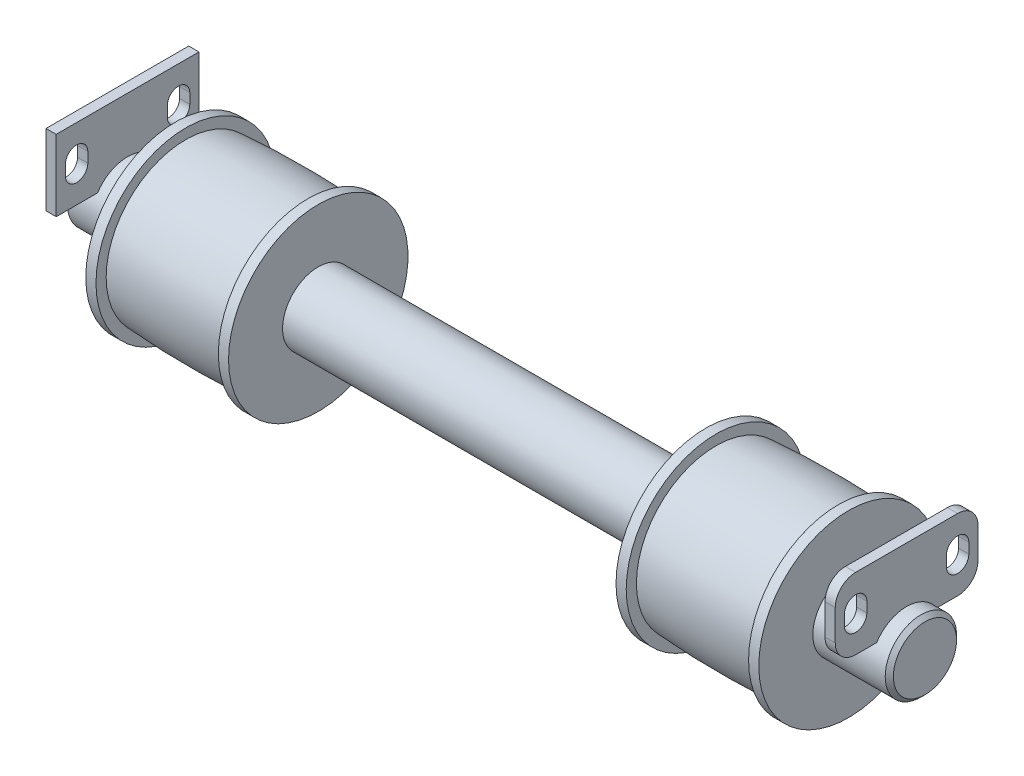
from build123d import *

# Parameters (mm, degrees)
CUT_EXTRUDE_1_DEPTH      = 72379.34823682
CUT_EXTRUDE_1_DEPTH_BACK = 72379.34823682
SKETCH_2_W               = 5
SKETCH_2_H               = 25.766795942
SKETCH_3_W               = 5
SKETCH_3_H               = 70
EXTRUDE_1_DEPTH          = 35
EXTRUDE_1_2_DEPTH        = 35
FILLET_1_R               = 10
CUT_EXTRUDE_2_DEPTH      = 4056.222125419
CUT_EXTRUDE_2_DEPTH_BACK = 4056.222125419


with BuildPart() as part:
    # 草图1 → 旋转1 (revolve)
    with BuildSketch(Plane.XY, mode=Mode.PRIVATE) as revolve_1_sk:
        with BuildLine():
            Line((72263.740728259, -3974.100882952), (72228.240728259, -3974.100882952))
            Line((72228.240728259, -3974.100882952), (72228.240728259, -3947.600882952))
            Line((72228.240728259, -3947.600882952), (72223.240728259, -3947.600882952))
            Line((72223.240728259, -3947.600882952), (72223.240728258, -3952.600882952))
            ThreePointArc((72223.240728258, -3952.600882952), (72193.240728259, -3951.600882952), (72163.240728259, -3952.600882952))
            Line((72163.240728259, -3952.600882952), (72163.240728259, -3947.600882952))
            Line((72163.240728259, -3947.600882952), (72158.240728259, -3947.600882952))
            Line((72158.240728259, -3947.600882952), (72158.240728259, -3974.100882952))
            Line((72158.240728259, -3974.100882952), (71968.240728259, -3974.100882952))
            Line((71968.240728259, -3974.100882952), (71968.240728259, -3947.600882952))
            Line((71968.240728259, -3947.600882952), (71963.240728259, -3947.600882952))
            Line((71963.240728259, -3947.600882952), (71963.240728258, -3952.600882952))
            ThreePointArc((71963.240728258, -3952.600882952), (71933.240728259, -3951.600882952), (71903.240728259, -3952.600882952))
            Line((71903.240728259, -3952.600882952), (71903.240728259, -3947.600882952))
            Line((71903.240728259, -3947.600882952), (71898.240728259, -3947.600882952))
            Line((71898.240728259, -3947.600882952), (71898.240728259, -3974.100882952))
            Line((71898.240728259, -3974.100882952), (71862.740728259, -3974.100882952))
            Line((71862.740728259, -3974.100882952), (71860.740728259, -3976.100882952))
            Line((71860.740728259, -3976.100882952), (71860.740728259, -3991.600882952))
            Line((71860.740728259, -3991.600882952), (72265.740728259, -3991.600882952))
            Line((72265.740728259, -3991.600882952), (72265.740728259, -3976.100882952))
            Line((72265.740728259, -3976.100882952), (72263.740728259, -3974.100882952))
        make_face()
    revolve(revolve_1_sk.sketch.rotate(Axis((71860.740728259, -3991.600882952, 0), (1, 0, 0)), 90), axis=Axis((71860.740728259, -3991.600882952, 0), (1, 0, 0)))

    # 草图2 → 切除-拉伸1 (cut, two sides: drawn at the far end of the back side and taken through both)
    with BuildSketch(Plane.XY.offset(-CUT_EXTRUDE_1_DEPTH_BACK)):
        with Locations((72254.240728259, -3969.217484981)):
            Rectangle(SKETCH_2_W, SKETCH_2_H)
        with Locations((71872.240728259, -3969.217484981)):
            Rectangle(SKETCH_2_W, SKETCH_2_H)
    extrude(amount=CUT_EXTRUDE_1_DEPTH + CUT_EXTRUDE_1_DEPTH_BACK, mode=Mode.SUBTRACT)


with BuildPart() as body_2:
    # 草图3 → 凸台-拉伸1 (new body)
    with BuildSketch(Plane(origin=(0, -3982.100882952, 0), x_dir=(1, 0, 0), z_dir=(0, 1, 0))):
        with Locations((72254.240728259, 0)):
            Rectangle(SKETCH_3_W, SKETCH_3_H)
    extrude(amount=EXTRUDE_1_DEPTH)

    # 圆角1
    fillet_1_edges = [body_2.edges().sort_by_distance(p)[0] for p in [
        (72254.240728259, -3947.100882952, -35),
        (72254.240728259, -3982.100882952, -35),
        (72254.240728259, -3982.100882952, 35),
        (72254.240728259, -3947.100882952, 35),
    ]]
    fillet(fillet_1_edges, radius=FILLET_1_R)


with BuildPart() as body_3:
    # 草图3 → Extrude 1 2 (new body)
    with BuildSketch(Plane(origin=(0, -3982.100882952, 0), x_dir=(1, 0, 0), z_dir=(0, 1, 0))):
        with Locations((71872.240728259, 0)):
            Rectangle(SKETCH_3_W, SKETCH_3_H)
    extrude(amount=EXTRUDE_1_2_DEPTH)


with BuildPart() as cut_extrude_2_tool:
    # 草图4 → 切除-拉伸2 (new, two sides: drawn at the far end of the back side and taken through both)
    with BuildSketch(Plane(origin=(72256.740728259, 0, 0), x_dir=(0, 0, -1), z_dir=(1, 0, 0)).offset(-CUT_EXTRUDE_2_DEPTH_BACK)):
        with BuildLine():
            Line((-19.5, -3962.100882952), (-19.5, -3967.100882952))
            ThreePointArc((-19.5, -3967.100882952), (-25, -3972.600882952), (-30.5, -3967.100882952))
            Line((-30.5, -3967.100882952), (-30.5, -3962.100882952))
            ThreePointArc((-30.5, -3962.100882952), (-25, -3956.600882952), (-19.5, -3962.100882952))
        make_face()
        with BuildLine():
            Line((19.5, -3962.100882952), (19.5, -3967.100882952))
            ThreePointArc((19.5, -3967.100882952), (25, -3972.600882952), (30.5, -3967.100882952))
            Line((30.5, -3967.100882952), (30.5, -3962.100882952))
            ThreePointArc((30.5, -3962.100882952), (25, -3956.600882952), (19.5, -3962.100882952))
        make_face()
    extrude(amount=CUT_EXTRUDE_2_DEPTH + CUT_EXTRUDE_2_DEPTH_BACK)


with BuildPart() as body_3_1:
    add(body_3.part)

    # 切除-拉伸2: cut by cut_extrude_2_tool
    add(cut_extrude_2_tool.part, mode=Mode.SUBTRACT)


with BuildPart() as body_2_1:
    add(body_2.part)

    # 切除-拉伸2: cut by cut_extrude_2_tool
    add(cut_extrude_2_tool.part, mode=Mode.SUBTRACT)


solid = Compound([part.part, body_3_1.part, body_2_1.part])
